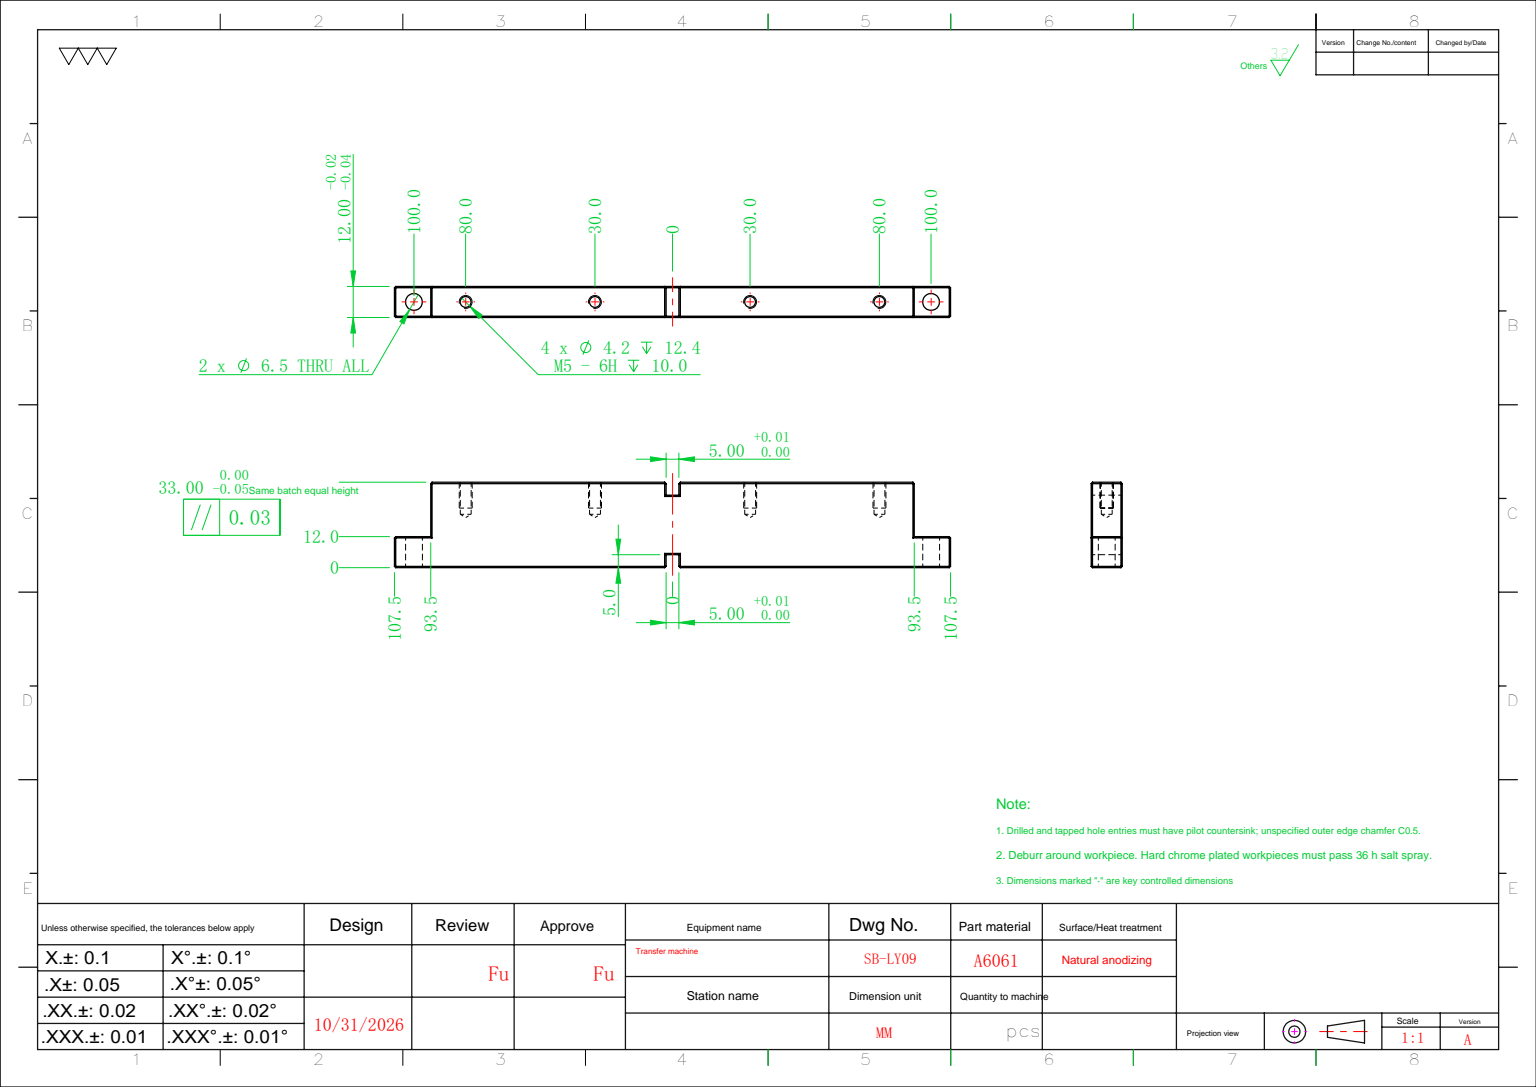
SolidWorks part; units mm, degrees
ref_plane "前视基准面" through (0, 0, 0) normal (0, 0, 1) x (1, 0, 0)
ref_plane "上视基准面" through (0, 0, 0) normal (0, 1, 0) x (1, 0, 0)
ref_plane "右视基准面" through (0, 0, 0) normal (1, 0, 0) x (0, 0, -1)
sketch "草图1" plane through (0, 0, 0) normal (0, 0, 1) x (1, 0, 0)
  line L1 (-93.5, -16.5) -> (93.5, -16.5)
  line L2 (-93.5, -16.5) -> (-93.5, 16.5)
  line L3 (-93.5, 16.5) -> (93.5, 16.5)
  line L4 (93.5, -16.5) -> (93.5, 16.5)
  line L5 (-93.5, -16.5) -> (93.5, 16.5) construction
  line L6 (-93.5, 16.5) -> (93.5, -16.5) construction
  point P0 (0, 0)
  dimension "D1" = 187
  dimension "D2" = 33
extrude "凸台-拉伸1" add sketch "草图1" along normal blind 12
hole_wizard "M5 螺纹孔1" positions "草图7" profile "草图5" tap size "M5" standard "ISO"
sketch "草图7" plane through (0, -16.5, 0) normal (0, -1, 0) x (-1, 0, 0)
  line L0 (93.5, -6) -> (-93.5, -6) construction
  line L1 (93.5, -12) -> (93.5, 0) construction
  line L2 (-93.5, -12) -> (-93.5, 0) construction
  line L4 (0, -12) -> (0, 0) construction
  line L5 (93.5, -12) -> (-93.5, -12) construction
  point P0 (-80, -6)
  point P3 (-30, -6)
  point P6 (30, -6)
  point P9 (80, -6)
  dimension "D1" = 60
  dimension "D2" = 160
sketch "草图5" plane through (80, -16.5, 6) normal (1, 0, 0) x (0, 0, -1)
  line L0 (0, 0) -> (0, 13.6618)
  line L1 (0, 13.6618) -> (2.1, 12.4)
  line L2 (2.1, 12.4) -> (2.1, 0)
  line L5 (2.1, 0) -> (0, 0)
  line L10 (0, 13.6618) -> (-2.1, 12.4) construction
  line L11 (0, -6.35) -> (0, 107.95) construction
  dimension "螺纹孔钻头直径" = 4.2
  dimension "螺纹孔钻头深度" = 12.4
  dimension "导头角度" = 118
cosmetic thread "孔螺蚊线1" parameters "D1"=10, "D2"=5
cosmetic thread "孔螺蚊线2" parameters "D1"=10, "D2"=5
cosmetic thread "孔螺蚊线3" parameters "D1"=10, "D2"=5
cosmetic thread "孔螺蚊线4" parameters "D1"=10, "D2"=5
sketch "草图8" plane through (0, -16.5, 0) normal (0, -1, 0) x (1, 0, 0)
  line L0 (-93.5, 0) -> (93.5, 0) construction
  line L1 (-2.5, 0) -> (2.5, 0)
  line L2 (-2.5, 0) -> (-2.5, 12)
  line L3 (-2.5, 12) -> (2.5, 12)
  line L4 (2.5, 0) -> (2.5, 12)
  line L5 (-93.5, 12) -> (93.5, 12) construction
  line L6 (0, 0) -> (0, 12) construction
  dimension "D1" = 5
extrude "切除-拉伸2" cut sketch "草图8" against normal blind 5
sketch "草图11" plane through (0, 0, 12) normal (0, 0, 1) x (1, 0, 0)
  line L0 (93.5, 16.5) -> (-93.5, 16.5) construction
  line L1 (-2.5, 16.5) -> (2.5, 16.5)
  line L2 (-2.5, 16.5) -> (-2.5, 11.5)
  line L3 (-2.5, 11.5) -> (2.5, 11.5)
  line L4 (2.5, 16.5) -> (2.5, 11.5)
  line L5 (0, 0) -> (0, 37.2706) construction
  line L6 (2.5, -11.5) -> (-2.5, -11.5) construction
  line L7 (-2.5, -11.5) -> (-2.5, -16.5) construction
extrude "切除-拉伸3" cut sketch "草图11" against normal through all
sketch "草图12" plane through (0, 0, 12) normal (0, 0, 1) x (1, 0, 0)
  line L0 (0, 0) -> (0, 31.6297) construction
  line L1 (93.5, 16.5) -> (107.5, 16.5)
  line L2 (93.5, 16.5) -> (93.5, 4.5)
  line L3 (93.5, 4.5) -> (107.5, 4.5)
  line L4 (107.5, 16.5) -> (107.5, 4.5)
  line L5 (-107.5, 16.5) -> (-107.5, 4.5)
  line L6 (-93.5, 4.5) -> (-107.5, 4.5)
  line L7 (-93.5, 16.5) -> (-93.5, 4.5)
  line L8 (-93.5, 16.5) -> (-107.5, 16.5)
  dimension "D1" = 12
  dimension "D2" = 215
extrude "凸台-拉伸2" add sketch "草图12" against normal up to surface (12 mm away) up to face at (0, 0, 0)
hole_wizard "Ø6.5 (6.5) 直径孔1" positions "草图13" profile "草图14" hole size "Ø6.5" standard "ISO" end condition through all
sketch "草图13" plane through (0, 4.5, 0) normal (0, -1, 0) x (-1, 0, 0)
  line L0 (0, 0) -> (0, -29.3397) construction
  line L2 (107.5, -6) -> (-107.5, -6) construction
  line L3 (107.5, 0) -> (107.5, -12) construction
  line L4 (-107.5, 0) -> (-107.5, -12) construction
  point P0 (-100, -6)
  point P8 (100, -6)
  dimension "D1" = 200
sketch "草图14" plane through (100, 4.5, 6) normal (1, 0, 0) x (0, 0, -1)
  line L0 (0, 0) -> (0, 12)
  line L1 (0, 12) -> (3.25, 12)
  line L2 (3.25, 12) -> (3.25, 0)
  line L5 (3.25, 0) -> (0, 0)
  line L11 (0, -6.35) -> (0, 107.95) construction
  dimension "通孔孔直径" = 6.5
  dimension "通孔孔深度" = 12
chamfer "倒角1" distance 0.5 angle 45 42 edges at (-2.5, 16.5, 6) (107.5, 16.5, 6) (2.5, 16.5, 6) (-55, 16.5, 12) (-55, 16.5, 0) (-100.5, 4.5, 0) (-93.5, -6, 0) (-93.5, -6, 12) (-48, -16.5, 0) (-48, -16.5, 12) (-2.5, -14, 0) (-2.5, -14, 12) (0, -11.5, 0) (0, -11.5, 12) (2.5, -14, 12) (2.5, -14, 0) (48, -16.5, 12) (48, -16.5, 0) (93.5, -6, 0) (93.5, -6, 12) (100.5, 4.5, 0) (-2.5, 14, 12) (-2.5, 14, 0) (0, 11.5, 12) (0, 11.5, 0) (2.5, 14, 12) (2.5, 14, 0) (55, 16.5, 0) (55, 16.5, 12) (107.5, 10.5, 0) (107.5, 10.5, 12) (107.5, 4.5, 6) (100.5, 4.5, 12) (93.5, -16.5, 6) (-107.5, 10.5, 12) (-107.5, 16.5, 6) (-107.5, 10.5, 0) (-107.5, 4.5, 6) (-100.5, 4.5, 12) (-93.5, -16.5, 6) (2.5, -16.5, 6) (-2.5, -16.5, 6)
